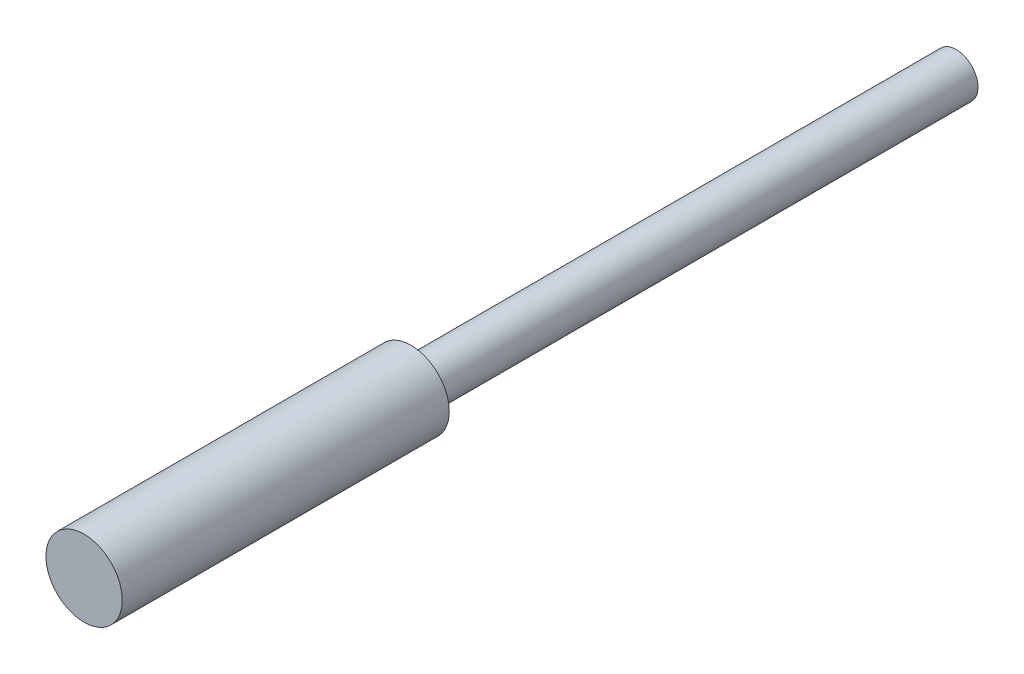
SolidWorks part; units mm, degrees
ref_plane "Front Plane" through (0, 0, 0) normal (0, 0, 1) x (1, 0, 0)
ref_plane "Top Plane" through (0, 0, 0) normal (0, 1, 0) x (1, 0, 0)
ref_plane "Right Plane" through (0, 0, 0) normal (1, 0, 0) x (0, 0, -1)
sketch "Sketch1" plane through (0, 0, 0) normal (0, 0, 1) x (1, 0, 0)
  circle A0 centre (0, 0) radius 1.4
  dimension "D1" = 2.8
extrude "Boss-Extrude1" add sketch "Sketch1" along normal blind 12
sketch "Sketch2" plane through (0, 0, 0) normal (0, 0, -1) x (-1, 0, 0)
  circle A0 centre (0, 0) radius 0.8
  dimension "D1" = 1.6
extrude "Boss-Extrude2" add sketch "Sketch2" along normal blind 20
